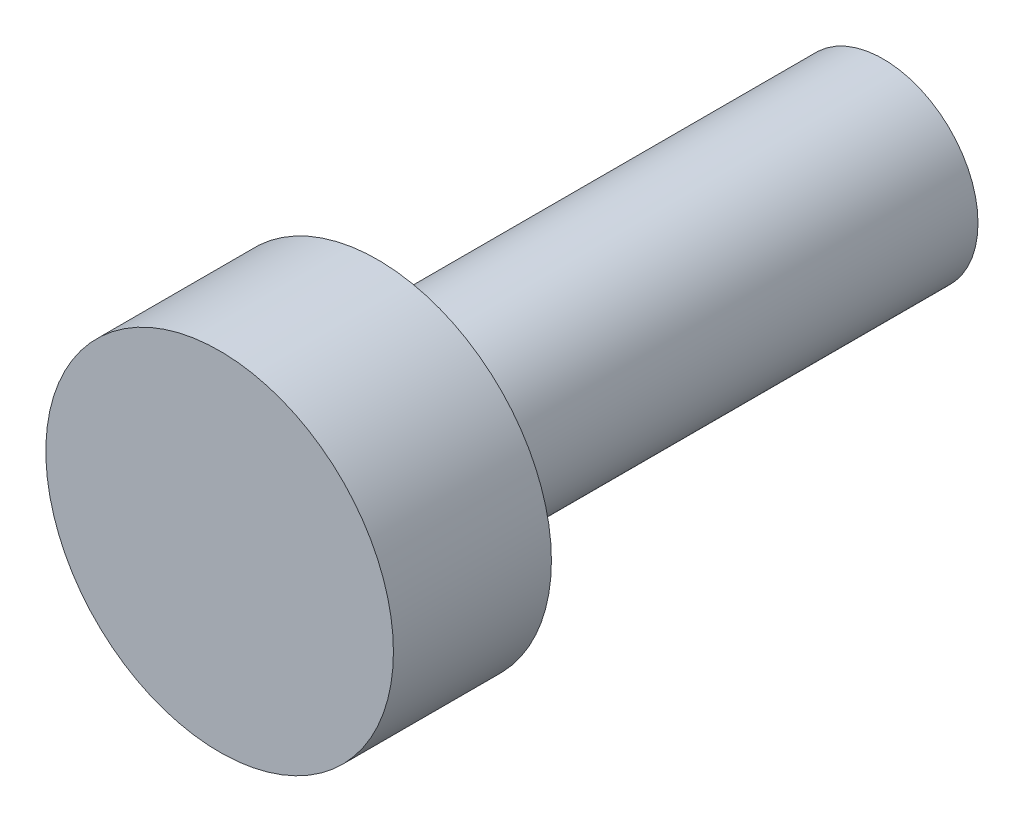
SolidWorks part; units mm, degrees
ref_plane "前视基准面" through (0, 0, 0) normal (0, 0, 1) x (1, 0, 0)
ref_plane "上视基准面" through (0, 0, 0) normal (0, 1, 0) x (1, 0, 0)
ref_plane "右视基准面" through (0, 0, 0) normal (1, 0, 0) x (0, 0, -1)
other "Configuration Table"
sketch "草图1" plane through (0, 0, 0) normal (0, 0, 1) x (1, 0, 0)
  circle A0 centre (0, 0) radius 1.5
  point P0 (0, 0)
  dimension "D1" = 3
extrude "凸台-拉伸1" add sketch "草图1" against normal blind 8
sketch "草图2" plane through (0, 0, 0) normal (0, 0, 1) x (1, 0, 0)
  circle A0 centre (0, 0) radius 2.75
  point P0 (0, 0)
  dimension "D1" = 5.5
extrude "凸台-拉伸2" add sketch "草图2" along normal blind 2.5
